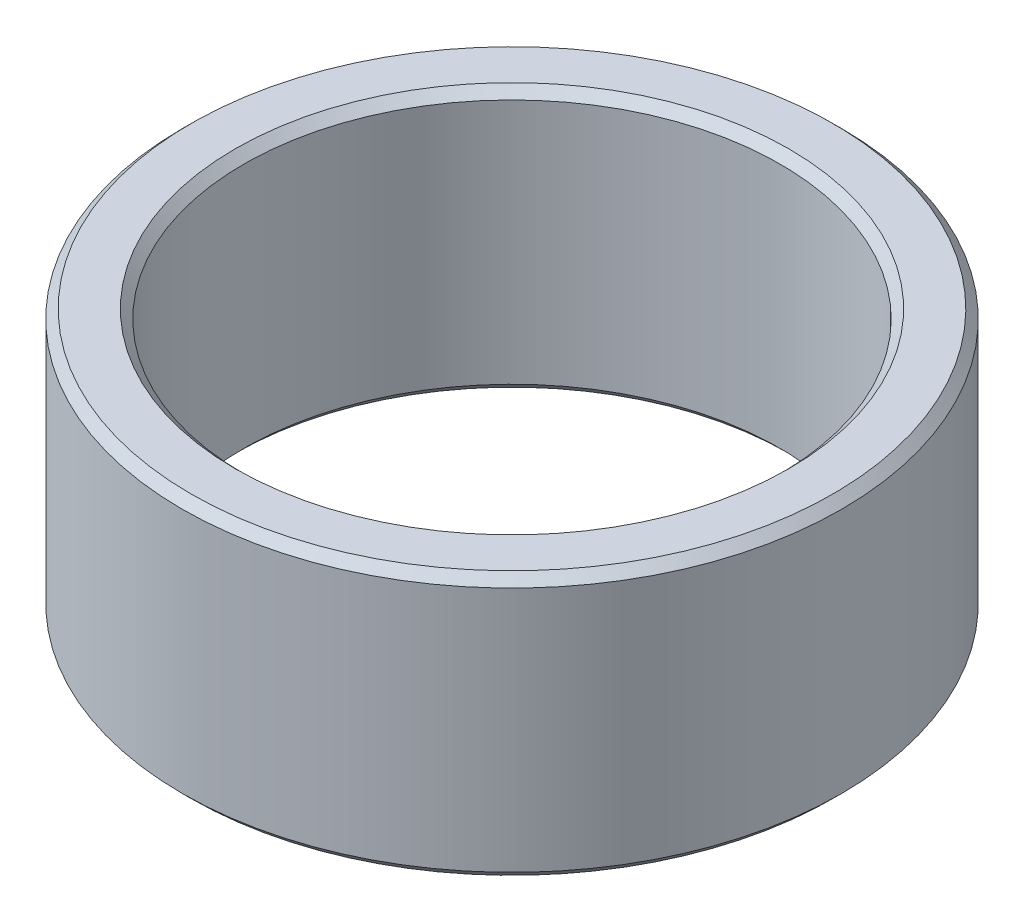
SolidWorks part; units mm, degrees
material "20 steel"
ref_plane "Front Plane" through (0, 0, 0) normal (0, 0, 1) x (1, 0, 0)
ref_plane "Top Plane" through (0, 0, 0) normal (0, 1, 0) x (1, 0, 0)
ref_plane "Right Plane" through (0, 0, 0) normal (1, 0, 0) x (0, 0, -1)
other "Configuration Table"
sketch "Sketch1" plane through (0, 0, 0) normal (0, 1, 0) x (1, 0, 0)
  circle A0 centre (0, 0) radius 37.5
  circle A1 centre (0, 0) radius 30.5
  dimension "D1" = 75
  dimension "D2" = 61
extrude "Boss-Extrude1" add sketch "Sketch1" along normal blind 30
chamfer "Chamfer1" distance 1 angle 45 4 edges at (0, 30, 37.5) (0, 0, 37.5) (0, 30, 30.5) (0, 0, 30.5)
